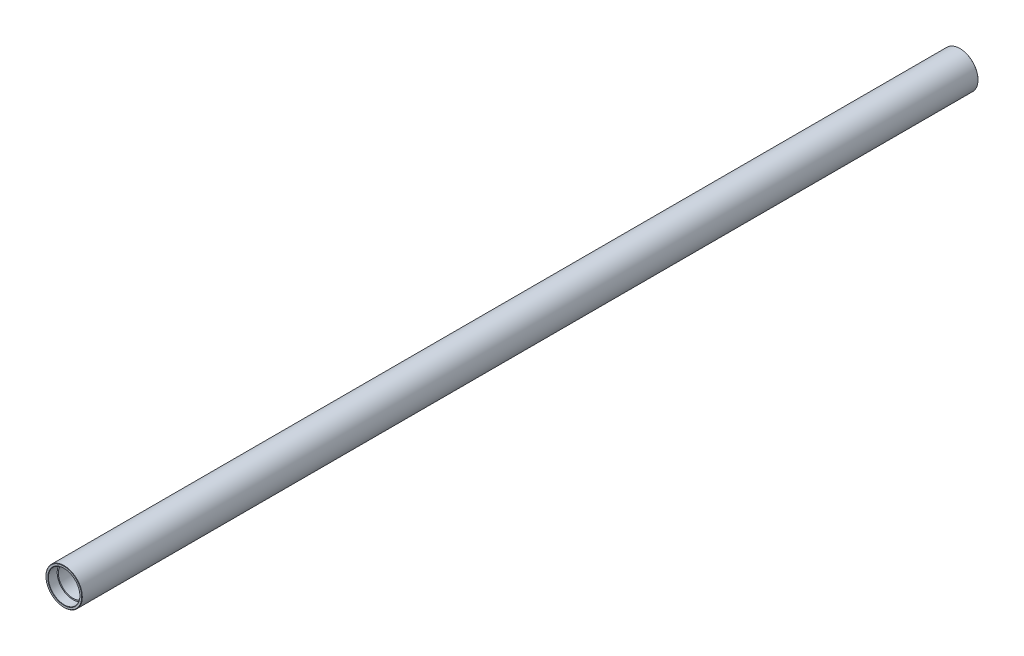
from build123d import *

# Parameters (mm, degrees)
SKETCH_1_R          = 30
EXTRUDE_1_DEPTH     = 1480
SKETCH_2_R          = 24
CUT_EXTRUDE_1_DEPTH = 1600
SKETCH_3_R          = 26
CUT_EXTRUDE_2_DEPTH = 15
CUT_EXTRUDE_START   = -15
SKETCH_4_R          = 26
CUT_EXTRUDE_3_DEPTH = 15
CHAMFER_1_SIZE      = 0.5


with BuildPart() as part:
    # 草图1 → 凸台-拉伸1 (new body)
    with BuildSketch(Plane.XY):
        Circle(SKETCH_1_R)
    extrude(amount=EXTRUDE_1_DEPTH)

    # 草图2 → 切除-拉伸1 (cut)
    with BuildSketch(Plane(origin=(0, 0, 0), x_dir=(-1, 0, 0), z_dir=(0, 0, -1))):
        Circle(SKETCH_2_R)
    extrude(amount=-CUT_EXTRUDE_1_DEPTH, mode=Mode.SUBTRACT)

    # 草图3 → 切除-拉伸2 (cut)
    with BuildSketch(Plane(origin=(0, 0, 0), x_dir=(-1, 0, 0), z_dir=(0, 0, -1))):
        Circle(SKETCH_3_R)
    extrude(amount=-CUT_EXTRUDE_2_DEPTH, mode=Mode.SUBTRACT)

    # 草图4 → 切除-拉伸3 (cut)
    with BuildSketch(Plane.XY.offset(1480).offset(CUT_EXTRUDE_START)):
        with Locations(Location((0, 0, 0), (0, 0, 180))):
            Circle(SKETCH_4_R)
    extrude(amount=CUT_EXTRUDE_3_DEPTH, mode=Mode.SUBTRACT)

    # 倒角1
    chamfer_1_edges = [part.edges().sort_by_distance(p)[0] for p in [
        (26, 0, 0),
        (-30, 0, 0),
        (26, 0, 1480),
        (-30, 0, 1480),
    ]]
    chamfer(chamfer_1_edges, length=CHAMFER_1_SIZE)


solid = part.part
